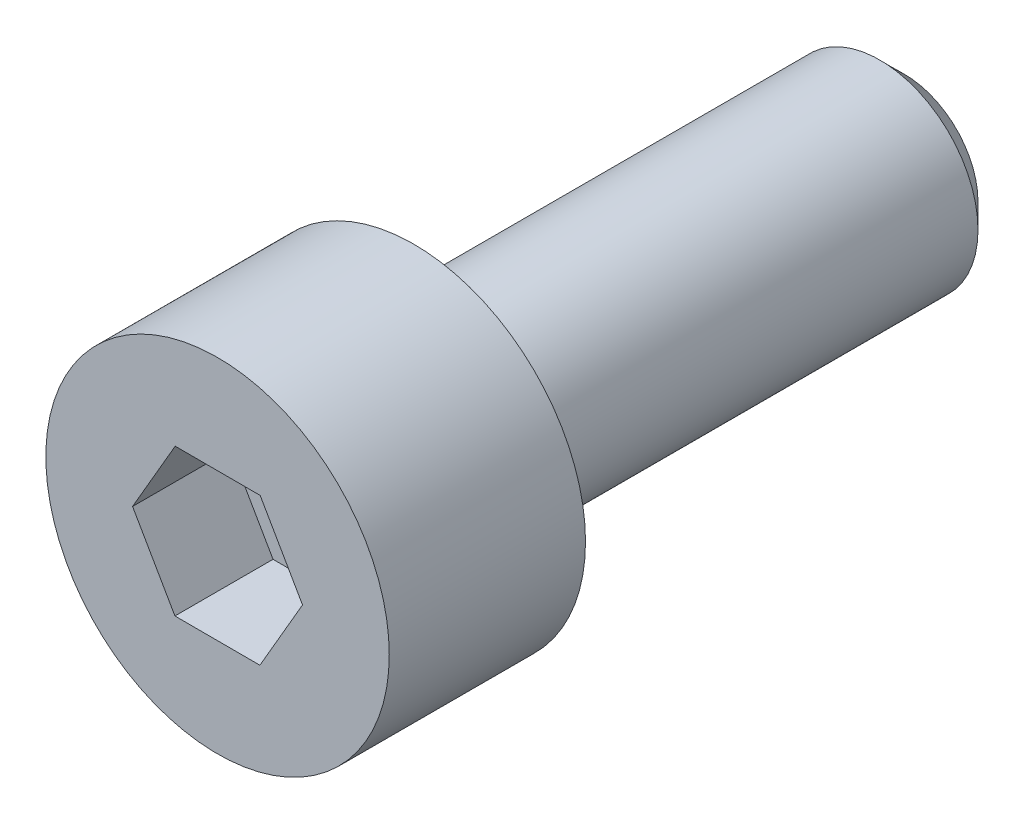
from build123d import *

# Parameters (mm, degrees)
SKETCH_1_R          = 2
EXTRUDE_1_DEPTH     = 10
SKETCH_2_R          = 3.5
EXTRUDE_2_DEPTH     = 4
CUT_EXTRUDE_1_DEPTH = 2
CHAMFER_1_SIZE      = 0.5
SKETCH_4_R          = 0.75
CUT_EXTRUDE_2_DEPTH = 13.980754986


with BuildPart() as part:
    # 草图1 → 凸台-拉伸1 (new body)
    with BuildSketch(Plane.XY):
        Circle(SKETCH_1_R)
    extrude(amount=EXTRUDE_1_DEPTH)

    # 草图2 → 凸台-拉伸2 (add)
    with BuildSketch(Plane.XY.offset(10)):
        Circle(SKETCH_2_R)
    extrude(amount=EXTRUDE_2_DEPTH)

    # 草图3 → 切除-拉伸1 (cut)
    with BuildSketch(Plane.XY.offset(14)):
        Polygon((-0.863155152, 1.501653483), (-1.73204764, 0.003312453), (-0.868892488, -1.498341031), (0.863155152, -1.501653483), (1.73204764, -0.003312453), (0.868892488, 1.498341031), align=None)
    extrude(amount=-CUT_EXTRUDE_1_DEPTH, mode=Mode.SUBTRACT)

    # 倒角1
    chamfer_1_edges = [part.edges().sort_by_distance(p)[0] for p in [
        (-2, 0, 0),
    ]]
    chamfer(chamfer_1_edges, length=CHAMFER_1_SIZE)

    # 草图4 → 切除-拉伸2 (cut, through all)
    with BuildSketch(Plane.XY.offset(12)):
        Circle(SKETCH_4_R)
    extrude(amount=-CUT_EXTRUDE_2_DEPTH, mode=Mode.SUBTRACT)


solid = part.part
